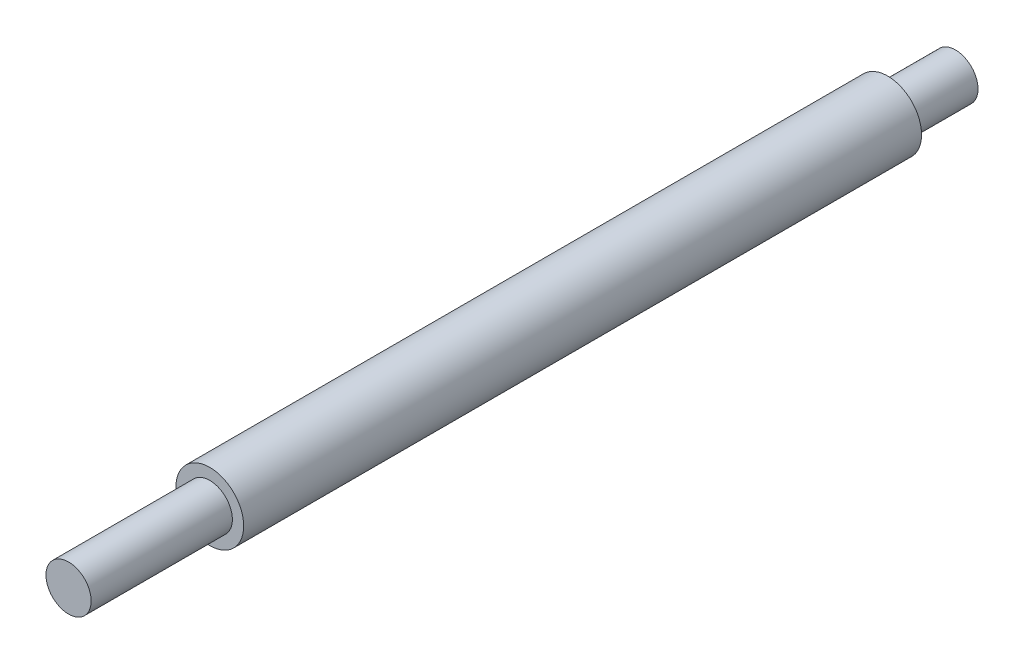
from build123d import *

# Parameters (mm, degrees)
SKETCH_1_R      = 6
EXTRUDE_1_DEPTH = 120
SKETCH_2_R      = 4
EXTRUDE_2_DEPTH = 12
EXTRUDE_START   = 25
SKETCH_3_R      = 4
EXTRUDE_3_DEPTH = 25


with BuildPart() as part:
    # 草图1 → 凸台-拉伸1 (new body)
    with BuildSketch(Plane.XY):
        Circle(SKETCH_1_R)
    extrude(amount=EXTRUDE_1_DEPTH)

    # 草图2 → 凸台-拉伸2 (add)
    with BuildSketch(Plane(origin=(0, 0, 0), x_dir=(-1, 0, 0), z_dir=(0, 0, -1))):
        Circle(SKETCH_2_R)
    extrude(amount=EXTRUDE_2_DEPTH)

    # 草图3 → 凸台-拉伸3 (add)
    with BuildSketch(Plane.XY.offset(120).offset(EXTRUDE_START)):
        with Locations(Location((0, 0, 0), (0, 0, 180))):
            Circle(SKETCH_3_R)
    extrude(amount=-EXTRUDE_3_DEPTH)


solid = part.part
